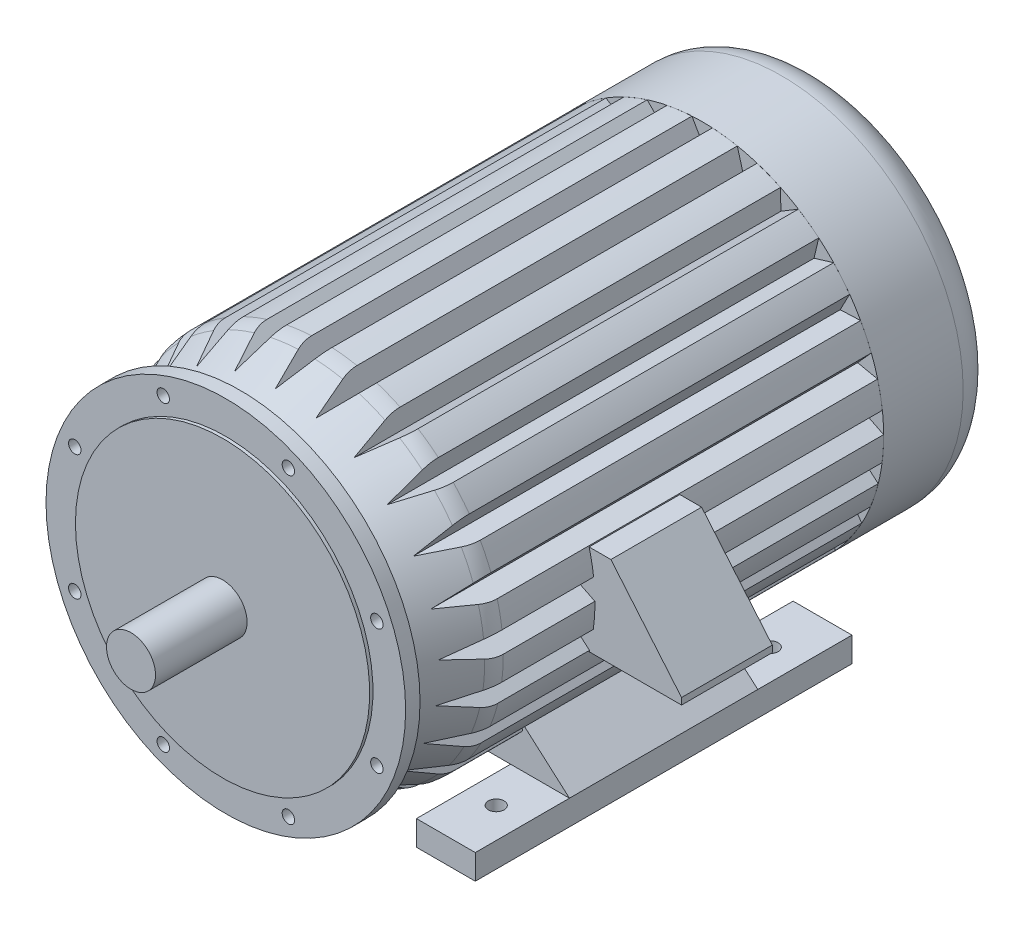
from build123d import *

# Parameters (mm, degrees)
SKETCH1_R          = 37.5
EXTRUDE1_DEPTH     = 140
SKETCH3_R          = 225
EXTRUDE2_DEPTH     = 5
SKETCH4_R          = 275
EXTRUDE3_DEPTH     = 22
EXTRUDE4_START     = -883
SKETCH5_R          = 277.5
EXTRUDE4_DEPTH     = 883
SKETCH7_OUTSIDE_W  = 1721.29
SKETCH7_OUTSIDE_H  = 1721.29
SKETCH7_OUTSIDE_R  = 225
CUT_EXTRUDE2_DEPTH = 967.282308645
CUT_EXTRUDE2_DRAFT = 25
SKETCH6_R          = 9.5
CUT_EXTRUDE1_DEPTH = 22
CIRPATTERN1_COUNT  = 8
FILLET1_R          = 55
SKETCH8_R          = 277.6
EXTRUDE5_DEPTH     = 121.6
CUT_EXTRUDE3_DEPTH = 696.4
CIRPATTERN2_COUNT  = 25
SKETCH10_W         = 138.75
SKETCH10_H         = 138.75
EXTRUDE6_DEPTH     = 410
CHAMFER1_SIZE      = 128.75
CHAMFER1_SIZE2     = 108.034077514
SKETCH11_W         = 90
SKETCH11_H         = 576
SKETCH11_R         = 12
EXTRUDE7_DEPTH     = 38
EXTRUDE7_2_DEPTH   = 38
EXTRUDE8_DEPTH     = 144


with BuildPart() as part:
    # Sketch1 → Extrude1 (new body)
    with BuildSketch(Plane.XY):
        Circle(SKETCH1_R)
    extrude(amount=-EXTRUDE1_DEPTH)

    # Sketch3 → Extrude2 (add)
    with BuildSketch(Plane(origin=(0, 0, -140), x_dir=(-1, 0, 0), z_dir=(0, 0, -1))):
        Circle(SKETCH3_R)
    extrude(amount=EXTRUDE2_DEPTH)

    # Sketch4 → Extrude3 (add)
    with BuildSketch(Plane(origin=(0, 0, -145), x_dir=(-1, 0, 0), z_dir=(0, 0, -1))):
        Circle(SKETCH4_R)
    extrude(amount=EXTRUDE3_DEPTH)

    # Sketch5 → Extrude4 (add)
    with BuildSketch(Plane.XY.offset(-167).offset(EXTRUDE4_START)):
        Circle(SKETCH5_R)
    extrude(amount=EXTRUDE4_DEPTH)


with BuildPart() as cut_extrude2_tool:
    # Sketch7 outside → Cut-Extrude2 (with draft: the straight prism first)
    with BuildSketch(Plane(origin=(0, 0, -167), x_dir=(-1, 0, 0), z_dir=(0, 0, -1))):
        Rectangle(SKETCH7_OUTSIDE_W, SKETCH7_OUTSIDE_H)
        Circle(SKETCH7_OUTSIDE_R, mode=Mode.SUBTRACT)
    extrude(amount=CUT_EXTRUDE2_DEPTH)
    # Cut-Extrude2: the draft: its side faces are tilted about the plane it starts from
    cut_extrude2_sides = [cut_extrude2_tool.faces().sort_by_distance(p)[0] for p in [
        (0, -860.645, -650.641154322),
        (-860.645, 0, -650.641154322),
        (0, 860.645, -650.641154322),
        (860.645, 0, -650.641154322),
        (225, 0, -650.641154322),
    ]]
    draft(cut_extrude2_sides, Plane(origin=(0, 0, -167), x_dir=(-1, 0, 0), z_dir=(0, 0, -1)), CUT_EXTRUDE2_DRAFT)


with BuildPart() as part_1:
    add(part.part)

    # Cut-Extrude2: cut by cut_extrude2_tool
    add(cut_extrude2_tool.part, mode=Mode.SUBTRACT)

    # Sketch6 → Cut-Extrude1 (cut)
    with BuildSketch(Plane.XY.offset(-145)):
        with Locations((-95.670858091, 230.969883128)):
            Circle(SKETCH6_R)
    cut_extrude1 = extrude(amount=-CUT_EXTRUDE1_DEPTH, mode=Mode.SUBTRACT)

    # CirPattern1: Cut-Extrude1 ×8 about axis
    cirpattern1_axis = Axis((0, 0, 0), (0, 0, 1))
    for i in range(1, CIRPATTERN1_COUNT):
        add(cut_extrude1.rotate(cirpattern1_axis, i * 360 / CIRPATTERN1_COUNT), mode=Mode.SUBTRACT)

    # Fillet1
    fillet1_edges = [part_1.edges().sort_by_distance(p)[0] for p in [
        (-277.5, 0, -1050),
        (0, -277.5, -279.586613327),
    ]]
    fillet(fillet1_edges, radius=FILLET1_R)

    # Sketch8 → Extrude5 (add)
    with BuildSketch(Plane(origin=(0, 0, -873.4), x_dir=(-1, 0, 0), z_dir=(0, 0, -1))):
        with Locations(Location((0, 0, 0), (0, 0, 180))):
            Circle(SKETCH8_R)
    extrude(amount=EXTRUDE5_DEPTH)

    # Sketch9 → Cut-Extrude3 (cut)
    with BuildSketch(Plane(origin=(0, 0, -873.4), x_dir=(-1, 0, 0), z_dir=(0, 0, -1))):
        Polygon((0, 250), (23.815698604, 291.25), (-23.815698604, 291.25), align=None)
    cut_extrude3 = extrude(amount=-CUT_EXTRUDE3_DEPTH, mode=Mode.SUBTRACT)

    # CirPattern2: Cut-Extrude3 ×25 about axis
    cirpattern2_axis = Axis((0, 0, 0), (0, 0, 1))
    for i in range(1, CIRPATTERN2_COUNT):
        add(cut_extrude3.rotate(cirpattern2_axis, i * 360 / CIRPATTERN2_COUNT), mode=Mode.SUBTRACT)

    # Sketch10 → Extrude6 (add)
    with BuildSketch(Plane(origin=(0, 0, 0), x_dir=(0, 0, -1), z_dir=(1, 0, 0))):
        with Locations((501.275, 0)):
            Rectangle(SKETCH10_W, SKETCH10_H)
    extrude(amount=EXTRUDE6_DEPTH)

    # Chamfer1
    chamfer1_edges = [part_1.edges().sort_by_distance(p)[0] for p in [
        (410, 69.375, -501.275),
    ]]
    chamfer1_side = [part_1.faces().sort_by_distance(p)[0] for p in [
        (410, 0, -501.275),
    ]]
    chamfer(chamfer1_edges, length=CHAMFER1_SIZE, length2=CHAMFER1_SIZE2, reference=chamfer1_side[0])



with BuildPart() as body_2:
    # Sketch11 → Extrude7 (new body)
    with BuildSketch(Plane(origin=(0, -280, 0), x_dir=(-1, 0, 0), z_dir=(0, 1, 0))):
        with Locations((230, -539.5)):
            Rectangle(SKETCH11_W, SKETCH11_H)
        with Locations(Location((228.5, -749, 0), (0, 0, 90))):
            Circle(SKETCH11_R, mode=Mode.SUBTRACT)
        with Locations(Location((228.5, -330, 0), (0, 0, 270))):
            Circle(SKETCH11_R, mode=Mode.SUBTRACT)
    extrude(amount=EXTRUDE7_DEPTH)


with BuildPart() as body_3:
    # Sketch11 → Extrude7 2 (new body)
    with BuildSketch(Plane(origin=(0, -280, 0), x_dir=(-1, 0, 0), z_dir=(0, 1, 0))):
        with Locations((-230, -539.5)):
            Rectangle(SKETCH11_W, SKETCH11_H)
        with Locations(Location((-228.5, -330, 0), (0, 0, 90))):
            Circle(SKETCH11_R, mode=Mode.SUBTRACT)
        with Locations(Location((-228.5, -749, 0), (0, 0, 270))):
            Circle(SKETCH11_R, mode=Mode.SUBTRACT)
    extrude(amount=EXTRUDE7_2_DEPTH)


with BuildPart() as part_2:
    add(part_1.part)

    add(body_2.part)  # Extrude8 merges body 2

    add(body_3.part)  # Extrude8 merges body 3
    # Sketch12 → Extrude8 (add, symmetric)
    with BuildSketch(Plane.XY.offset(-539.5)):
        Polygon((275, -242), (0, 0), (-275, -242), align=None)
    extrude(amount=EXTRUDE8_DEPTH, both=True)


solid = part_2.part
